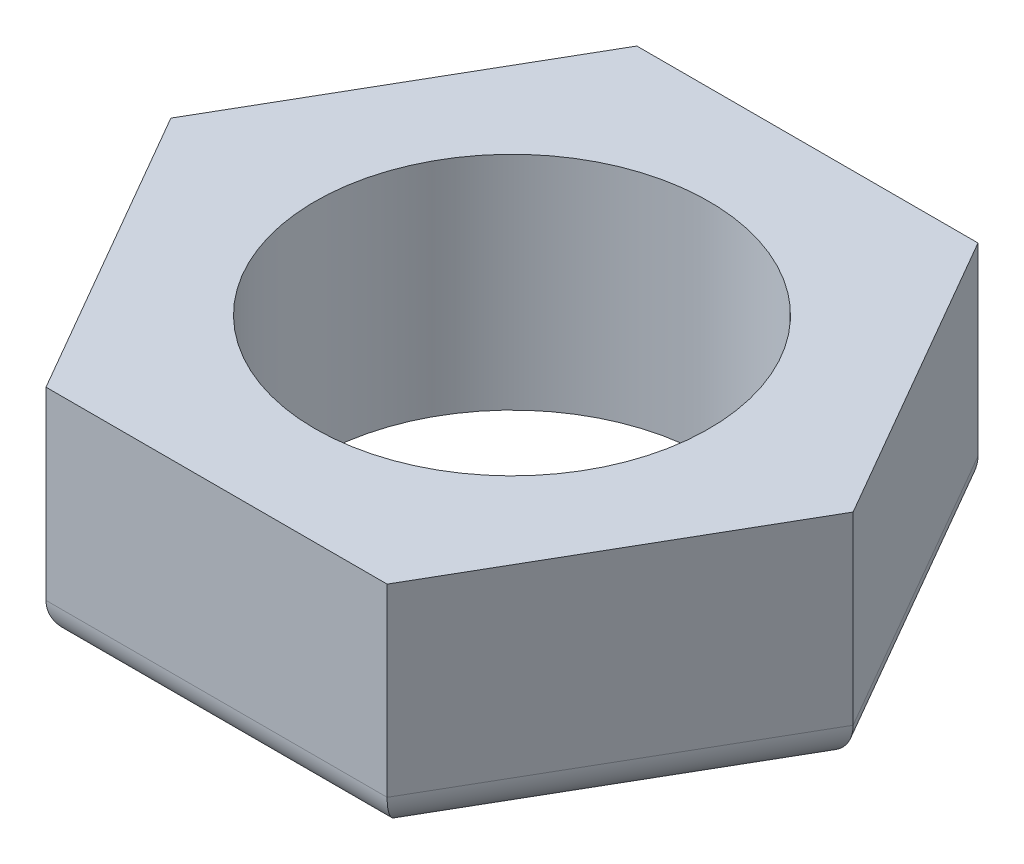
from build123d import *

# Parameters (mm, degrees)
SKETCH1_R      = 8
EXTRUDE1_DEPTH = 9
FILLET1_R      = 1.5


with BuildPart() as part:
    # Sketch1 → Extrude1 (new body)
    with BuildSketch(Plane(origin=(0, 0, 0), x_dir=(1, 0, 0), z_dir=(0, 1, 0))):
        Polygon((13.856406461, 0), (6.92820323, 12), (-6.92820323, 12), (-13.856406461, 0), (-6.92820323, -12), (6.92820323, -12), align=None)
        with Locations(Location((0, 0, 0), (0, 0, 270))):
            Circle(SKETCH1_R, mode=Mode.SUBTRACT)
    extrude(amount=EXTRUDE1_DEPTH)

    # Fillet1
    fillet1_edges = [part.edges().sort_by_distance(p)[0] for p in [
        (0, 0, 12),
        (-10.392304845, 0, 6),
        (-10.392304845, 0, -6),
        (0, 0, -12),
        (10.392304845, 0, -6),
        (10.392304845, 0, 6),
    ]]
    fillet(fillet1_edges, radius=FILLET1_R)


solid = part.part
